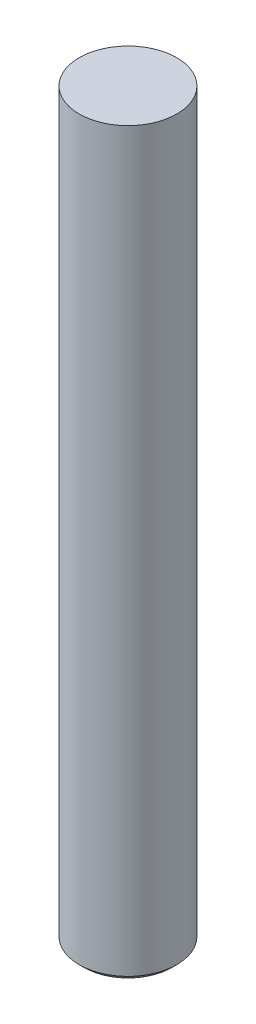
from build123d import *

# Parameters (mm, degrees)
SKETCH1_R           = 10
BOSS_EXTRUDE1_DEPTH = 76
CHAMFER1_SIZE       = 1


with BuildPart() as part:
    # Sketch1 → Boss-Extrude1 (new, symmetric)
    with BuildSketch(Plane(origin=(0, 0, 0), x_dir=(1, 0, 0), z_dir=(0, 1, 0))):
        with Locations(Location((0, 0, 0), (0, 0, 270))):
            Circle(SKETCH1_R)
    extrude(amount=BOSS_EXTRUDE1_DEPTH, both=True)

    # Chamfer1
    chamfer1_edges = [part.edges().sort_by_distance(p)[0] for p in [
        (0, -76, -10),
    ]]
    chamfer(chamfer1_edges, length=CHAMFER1_SIZE)


solid = part.part
